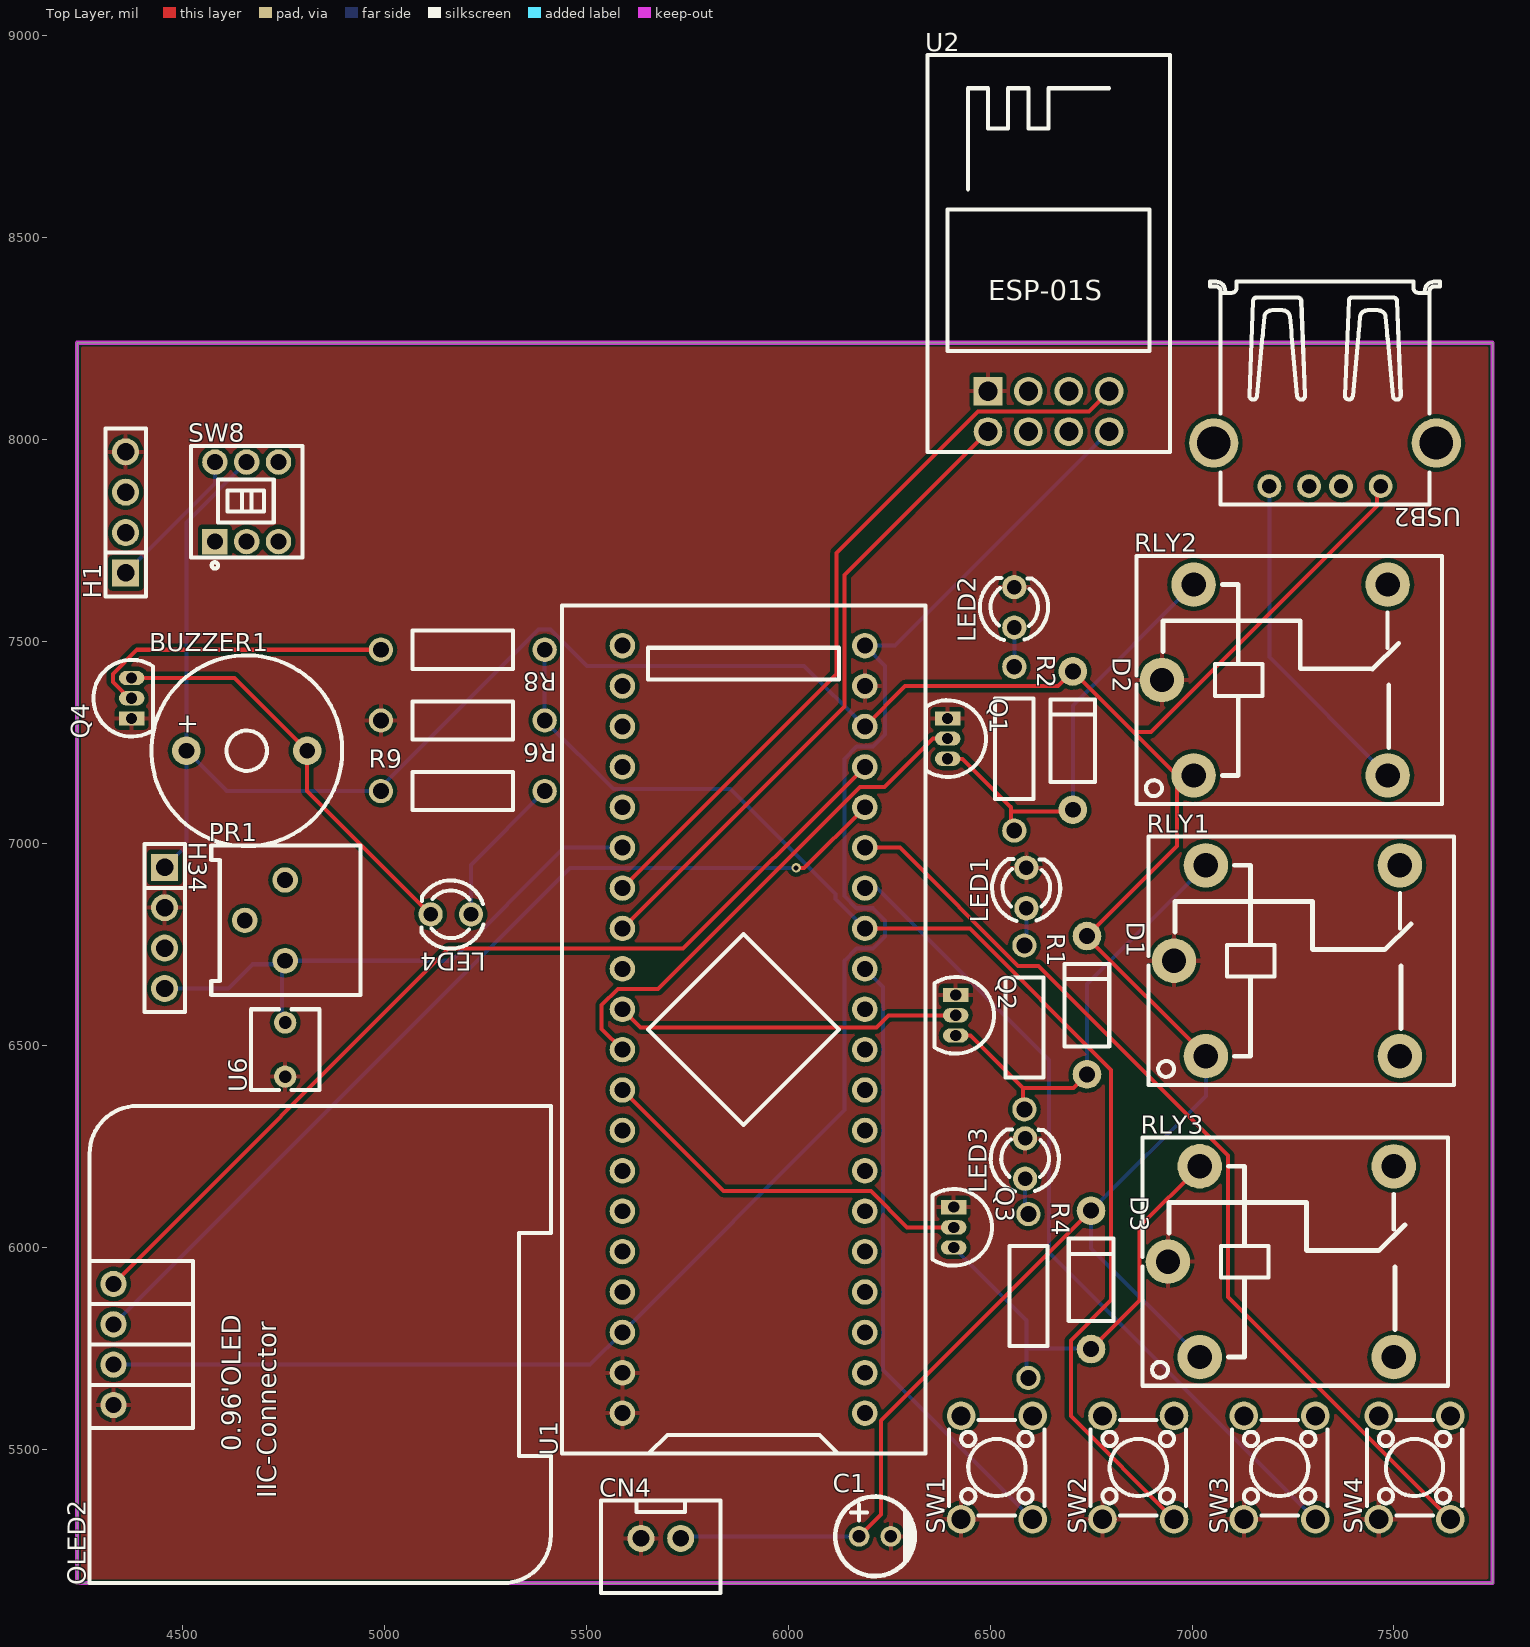
[diagram p0: Top Layer view]
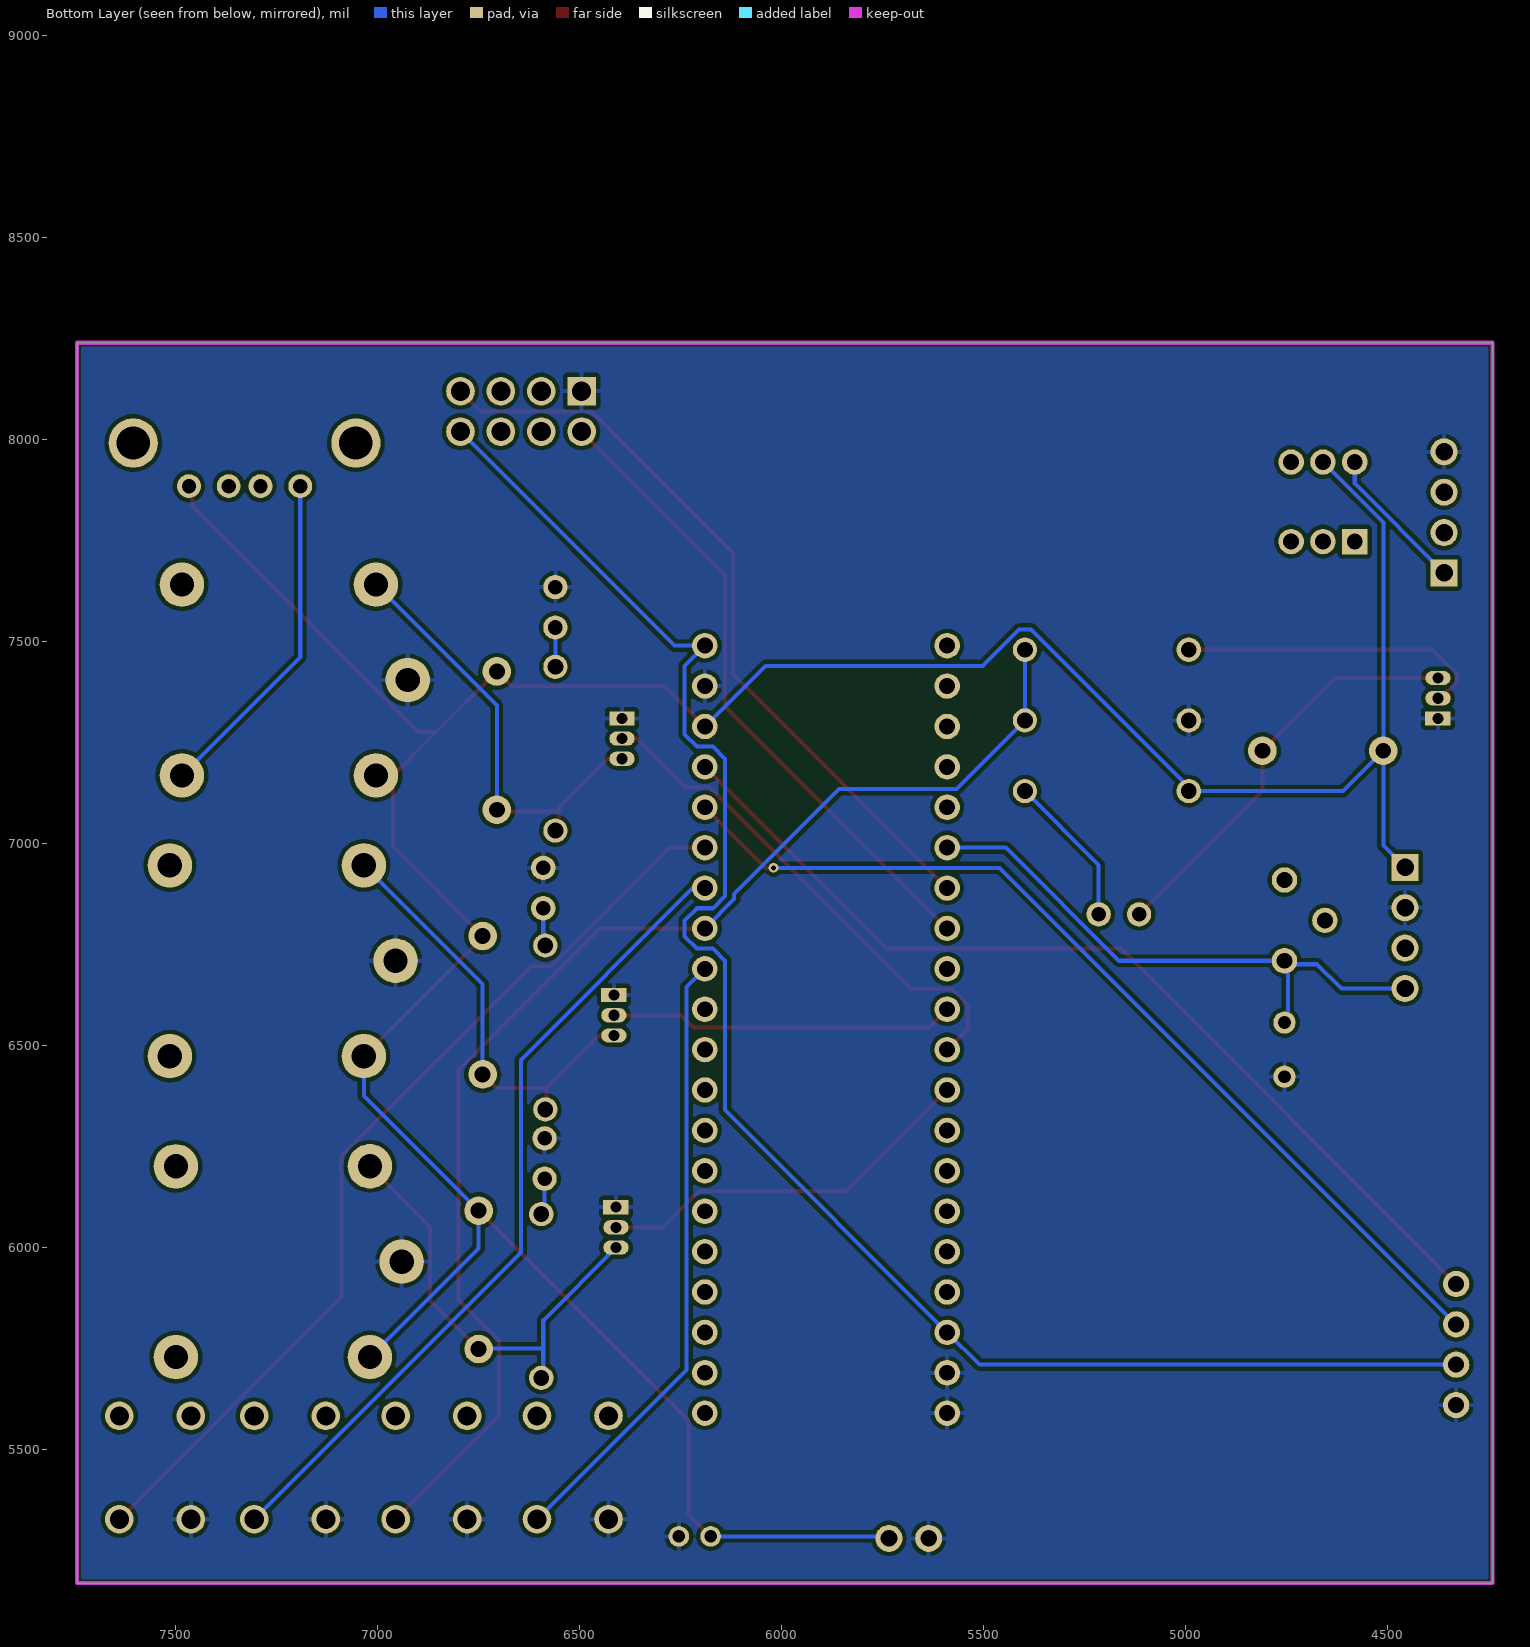
[diagram p1: Bottom Layer view, seen from below]
# Altium PCB MISC51908.pcbdoc
Units mil, origin at the board's own origin, x right, y up, seen from the top; angles counter-clockwise.
Board outline 3503.94 x 3070.87 mil, 2 copper layers (Top Layer, Bottom Layer), stack 62.206 mil thick; 36 components, 50 nets, 152 pads, 1 vias.

## Layer stack, top to bottom
Top Solder Mask Layer: solder mask 0.394, Dk 3.3
Top Layer: signal copper 1.379
Dielectric1: surface 59.449, FR4, Dk 4.5
Bottom Layer: signal copper 1.378
Bottom Solder Mask Layer: solder mask 0.394, Dk 3.3

## Board outline
4240,8240 4240,5169.13 7743.94,5169.13 7743.94,8240

## Design rules (kind name [scope] priority, off if disabled: settings)
BoardOutlineClearance copperThickness2oz_1 [All] p2 off: genericclearance=7.99 ignorepadtopadclearanceinfootprint=FALSE except(0: Arc-SplitContinuation Track-SplitContinuation SMDPad-SplitContinuation THPad-SplitContinuation Via-SplitContinuation Fill-SplitContinuation Region-SplitContinuation Poly-SplitContinuation Text-SplitContinuation Hole-SplitContinuation; 5.98: Arc-CutoutEdge Track-CutoutEdge SMDPad-CutoutEdge THPad-CutoutEdge Via-CutoutEdge Text-CutoutEdge; 6.9: Hole-OutlineEdge Hole-CutoutEdge; 10: Poly-OutlineEdge Poly-CutoutEdge; 11.81: Arc-OutlineEdge Track-OutlineEdge SMDPad-OutlineEdge THPad-OutlineEdge Via-OutlineEdge Fill-OutlineEdge Region-OutlineEdge Text-OutlineEdge Fill-CutoutEdge Region-CutoutEdge)
BoardOutlineClearance Plane_innerPlane_1 [All] p4 off: genericclearance=4.02 ignorepadtopadclearanceinfootprint=FALSE except(0: Arc-SplitContinuation Track-SplitContinuation SMDPad-SplitContinuation THPad-SplitContinuation Via-SplitContinuation Fill-SplitContinuation Region-SplitContinuation Poly-SplitContinuation Text-SplitContinuation Hole-SplitContinuation; 5.98: Arc-CutoutEdge Track-CutoutEdge SMDPad-CutoutEdge THPad-CutoutEdge Via-CutoutEdge Text-CutoutEdge; 6.9: Hole-OutlineEdge Hole-CutoutEdge; 10: Poly-OutlineEdge Poly-CutoutEdge; 11.81: Arc-OutlineEdge Track-OutlineEdge SMDPad-OutlineEdge THPad-OutlineEdge Via-OutlineEdge Fill-OutlineEdge Region-OutlineEdge Text-OutlineEdge Fill-CutoutEdge Region-CutoutEdge)
BoardOutlineClearance Copper_copperRegion_1 [All] p6 off: genericclearance=4.02 ignorepadtopadclearanceinfootprint=FALSE except(0: Arc-SplitContinuation Track-SplitContinuation SMDPad-SplitContinuation THPad-SplitContinuation Via-SplitContinuation Fill-SplitContinuation Region-SplitContinuation Poly-SplitContinuation Text-SplitContinuation Hole-SplitContinuation; 5.98: Arc-CutoutEdge Track-CutoutEdge SMDPad-CutoutEdge THPad-CutoutEdge Via-CutoutEdge Text-CutoutEdge; 6.9: Hole-OutlineEdge Hole-CutoutEdge; 10: Poly-OutlineEdge Poly-CutoutEdge; 11.81: Arc-OutlineEdge Track-OutlineEdge SMDPad-OutlineEdge THPad-OutlineEdge Via-OutlineEdge Fill-OutlineEdge Region-OutlineEdge Text-OutlineEdge Fill-CutoutEdge Region-CutoutEdge)
BoardOutlineClearance Copper_copperRegion_copperThickness1oz_1 [All] p8 off: genericclearance=4.02 ignorepadtopadclearanceinfootprint=FALSE except(0: Arc-SplitContinuation Track-SplitContinuation SMDPad-SplitContinuation THPad-SplitContinuation Via-SplitContinuation Fill-SplitContinuation Region-SplitContinuation Poly-SplitContinuation Text-SplitContinuation Hole-SplitContinuation; 5.98: Arc-CutoutEdge Track-CutoutEdge SMDPad-CutoutEdge THPad-CutoutEdge Via-CutoutEdge Text-CutoutEdge; 6.9: Hole-OutlineEdge Hole-CutoutEdge; 10: Poly-OutlineEdge Poly-CutoutEdge; 11.81: Arc-OutlineEdge Track-OutlineEdge SMDPad-OutlineEdge THPad-OutlineEdge Via-OutlineEdge Fill-OutlineEdge Region-OutlineEdge Text-OutlineEdge Fill-CutoutEdge Region-CutoutEdge)
BoardOutlineClearance Copper_copperRegion_Copper_copperRegion_1 [All] p10 off: genericclearance=4.02 ignorepadtopadclearanceinfootprint=FALSE except(0: Arc-SplitContinuation Track-SplitContinuation SMDPad-SplitContinuation THPad-SplitContinuation Via-SplitContinuation Fill-SplitContinuation Region-SplitContinuation Poly-SplitContinuation Text-SplitContinuation Hole-SplitContinuation; 5.98: Arc-CutoutEdge Track-CutoutEdge SMDPad-CutoutEdge THPad-CutoutEdge Via-CutoutEdge Text-CutoutEdge; 6.9: Hole-OutlineEdge Hole-CutoutEdge; 10: Poly-OutlineEdge Poly-CutoutEdge; 11.81: Arc-OutlineEdge Track-OutlineEdge SMDPad-OutlineEdge THPad-OutlineEdge Via-OutlineEdge Fill-OutlineEdge Region-OutlineEdge Text-OutlineEdge Fill-CutoutEdge Region-CutoutEdge)
BoardOutlineClearance copperThickness1oz_1 [All] p12: genericclearance=4.02 ignorepadtopadclearanceinfootprint=FALSE except(0: Arc-SplitContinuation Track-SplitContinuation SMDPad-SplitContinuation THPad-SplitContinuation Via-SplitContinuation Fill-SplitContinuation Region-SplitContinuation Poly-SplitContinuation Text-SplitContinuation Hole-SplitContinuation; 5.98: Arc-CutoutEdge Track-CutoutEdge SMDPad-CutoutEdge THPad-CutoutEdge Via-CutoutEdge Text-CutoutEdge; 6.9: Hole-OutlineEdge Hole-CutoutEdge; 10: Poly-OutlineEdge Poly-CutoutEdge; 11.81: Arc-OutlineEdge Track-OutlineEdge SMDPad-OutlineEdge THPad-OutlineEdge Via-OutlineEdge Fill-OutlineEdge Region-OutlineEdge Text-OutlineEdge Fill-CutoutEdge Region-CutoutEdge)
Clearance copperThickness2oz [All] p1 off: gap=7.99 ignorepadtopadclearanceinfootprint=FALSE except(5.98: SMDPad-Track SMDPad-SMDPad THPad-Track SMDPad-THPad THPad-THPad Track-Via SMDPad-Via THPad-Via Via-Via Fill-SMDPad Region-SMDPad Fill-THPad Region-THPad Fill-Via Region-Via Fill-Fill Fill-Region Region-Region Arc-Track Arc-SMDPad Arc-THPad Arc-Via Fill-Arc Region-Arc Arc-Arc Text-Track SMDPad-Text Text-THPad Text-Via Fill-Text Region-Text Arc-Text Text-Text; 6.9: Hole-Track Hole-SMDPad Hole-THPad Hole-Via Fill-Hole Region-Hole Hole-Arc Hole-Text; 10: Poly-Track Poly-SMDPad Poly-THPad Poly-Via Poly-Fill Poly-Region Poly-Poly Poly-Arc Poly-Text Poly-Hole; 11.81: Fill-Track Region-Track)
Clearance Plane_innerPlane [All] p3 off: gap=4.02 ignorepadtopadclearanceinfootprint=FALSE except(5.98: SMDPad-Track SMDPad-SMDPad THPad-Track SMDPad-THPad THPad-THPad Track-Via SMDPad-Via THPad-Via Via-Via Fill-SMDPad Region-SMDPad Fill-THPad Region-THPad Fill-Via Region-Via Fill-Fill Fill-Region Region-Region Arc-Track Arc-SMDPad Arc-THPad Arc-Via Fill-Arc Region-Arc Arc-Arc Text-Track SMDPad-Text Text-THPad Text-Via Fill-Text Region-Text Arc-Text Text-Text; 6.9: Hole-Track Hole-SMDPad Hole-THPad Hole-Via Fill-Hole Region-Hole Hole-Arc Hole-Text; 10: Poly-Track Poly-SMDPad Poly-THPad Poly-Via Poly-Fill Poly-Region Poly-Poly Poly-Arc Poly-Text Poly-Hole; 11.81: Fill-Track Region-Track)
Clearance Copper_copperRegion [All] p5 off: gap=4.02 ignorepadtopadclearanceinfootprint=FALSE except(5.98: SMDPad-Track SMDPad-SMDPad THPad-Track SMDPad-THPad THPad-THPad Track-Via SMDPad-Via THPad-Via Via-Via Fill-SMDPad Region-SMDPad Fill-THPad Region-THPad Fill-Via Region-Via Fill-Fill Fill-Region Region-Region Arc-Track Arc-SMDPad Arc-THPad Arc-Via Fill-Arc Region-Arc Arc-Arc Text-Track SMDPad-Text Text-THPad Text-Via Fill-Text Region-Text Arc-Text Text-Text; 6.9: Hole-Track Hole-SMDPad Hole-THPad Hole-Via Fill-Hole Region-Hole Hole-Arc Hole-Text; 10: Poly-Track Poly-SMDPad Poly-THPad Poly-Via Poly-Fill Poly-Region Poly-Poly Poly-Arc Poly-Text Poly-Hole; 11.81: Fill-Track Region-Track)
Clearance Copper_copperRegion_copperThickness1oz [All] p7 off: gap=4.02 ignorepadtopadclearanceinfootprint=FALSE except(5.98: SMDPad-Track SMDPad-SMDPad THPad-Track SMDPad-THPad THPad-THPad Track-Via SMDPad-Via THPad-Via Via-Via Fill-SMDPad Region-SMDPad Fill-THPad Region-THPad Fill-Via Region-Via Fill-Fill Fill-Region Region-Region Arc-Track Arc-SMDPad Arc-THPad Arc-Via Fill-Arc Region-Arc Arc-Arc Text-Track SMDPad-Text Text-THPad Text-Via Fill-Text Region-Text Arc-Text Text-Text; 6.9: Hole-Track Hole-SMDPad Hole-THPad Hole-Via Fill-Hole Region-Hole Hole-Arc Hole-Text; 10: Poly-Track Poly-SMDPad Poly-THPad Poly-Via Poly-Fill Poly-Region Poly-Poly Poly-Arc Poly-Text Poly-Hole; 11.81: Fill-Track Region-Track)
Clearance Copper_copperRegion_Copper_copperRegion [All] p9 off: gap=4.02 ignorepadtopadclearanceinfootprint=FALSE except(5.98: SMDPad-Track SMDPad-SMDPad THPad-Track SMDPad-THPad THPad-THPad Track-Via SMDPad-Via THPad-Via Via-Via Fill-SMDPad Region-SMDPad Fill-THPad Region-THPad Fill-Via Region-Via Fill-Fill Fill-Region Region-Region Arc-Track Arc-SMDPad Arc-THPad Arc-Via Fill-Arc Region-Arc Arc-Arc Text-Track SMDPad-Text Text-THPad Text-Via Fill-Text Region-Text Arc-Text Text-Text; 6.9: Hole-Track Hole-SMDPad Hole-THPad Hole-Via Fill-Hole Region-Hole Hole-Arc Hole-Text; 10: Poly-Track Poly-SMDPad Poly-THPad Poly-Via Poly-Fill Poly-Region Poly-Poly Poly-Arc Poly-Text Poly-Hole; 11.81: Fill-Track Region-Track)
Clearance copperThickness1oz [All] p11: gap=4.02 ignorepadtopadclearanceinfootprint=FALSE except(5.98: SMDPad-Track SMDPad-SMDPad THPad-Track SMDPad-THPad THPad-THPad Track-Via SMDPad-Via THPad-Via Via-Via Fill-SMDPad Region-SMDPad Fill-THPad Region-THPad Fill-Via Region-Via Fill-Fill Fill-Region Region-Region Arc-Track Arc-SMDPad Arc-THPad Arc-Via Fill-Arc Region-Arc Arc-Arc Text-Track SMDPad-Text Text-THPad Text-Via Fill-Text Region-Text Arc-Text Text-Text; 6.9: Hole-Track Hole-SMDPad Hole-THPad Hole-Via Fill-Hole Region-Hole Hole-Arc Hole-Text; 10: Poly-Track Poly-SMDPad Poly-THPad Poly-Via Poly-Fill Poly-Region Poly-Poly Poly-Arc Poly-Text Poly-Hole; 11.81: Fill-Track Region-Track)
DiffPairsRouting differentialPair [All] p1: maxlimit=6 minlimit=6 mostfreqgap=6 toplayer_minwidth=5 toplayer_prefwidth=10 toplayer_maxwidth=100 toplayer_mingap=6 toplayer_prefgap=6 toplayer_maxgap=6 bottomlayer_minwidth=5 bottomlayer_prefwidth=10 bottomlayer_maxwidth=100 bottomlayer_mingap=6 bottomlayer_prefgap=6 bottomlayer_maxgap=6 maxuncoupledlength=10
HoleToHoleClearance otherClearance [All] p1: gap=11.81 allowstackedmicrovias=TRUE
Length netLength [All] p1: minlimit=0 maxlimit=0
PasteMaskExpansion pasteMaskExpansion [All] p1: expansion=0
PlaneConnect innerPlane [All] p1: planeconnectstyle=Relief reliefexpansion=20 reliefentries=4 reliefconductorwidth=10 reliefairgap=10
PolygonConnect copperRegion_copperThickness1oz [All] p1 off: connectstyle=Relief reliefconductorwidth=10 reliefentries=4 polygonreliefangle="90 Angle" airgapwidth=10 via.connectstyle=Relief via.reliefconductorwidth=10 via.reliefentries=4 via.polygonreliefangle="90 Angle" via.airgapwidth=10
PolygonConnect copperRegion_Copper_copperRegion [All] p2 off: connectstyle=Relief reliefconductorwidth=10 reliefentries=4 polygonreliefangle="90 Angle" airgapwidth=10 via.connectstyle=Relief via.reliefconductorwidth=10 via.reliefentries=4 via.polygonreliefangle="90 Angle" via.airgapwidth=10
PolygonConnect copperRegion [(InNet('GND'))] p3: connectstyle=Relief reliefconductorwidth=10 reliefentries=4 polygonreliefangle="90 Angle" airgapwidth=10 via.connectstyle=Relief via.reliefconductorwidth=10 via.reliefentries=4 via.polygonreliefangle="90 Angle" via.airgapwidth=10
RoutingVias viaSize [All] p1: holewidth=12.01 width=24.02 viastyle="Through Hole" minholewidth=11.81 minwidth=19.68 maxholewidth=248.03 maxwidth=393.7
SolderMaskExpansion solderMaskExpansion [IsVia] p1: expansion=-1000 istentingtop=TRUE
SolderMaskExpansion solderMaskExpansion [All] p2: expansion=2 istentingtop=FALSE
Width copperThickness2oz_2 [All] p1 off: maxlimit=100 minlimit=8 preferedwidth=10
Width copperThickness1oz_2 [All] p2: maxlimit=100 minlimit=5 preferedwidth=10

## Components (designator, comment, footprint, x,y, rotation, side; value= is the part's Value field where it differs from the comment)
BUZZER1 "2.3kHz" BUZ-TH_BD12.0-P7.60-D0.6-FD 4660,7230 r0 top
C1 "10uF" CAP-TH_BD5.0-P2.00-D0.8-FD-10UF50VC110GL 6215,5285 r0 top
CN4 "XH2.54*2P_Through-hole" CONN-TH_2P-P2.50-XH2.54-2P 5685,5280 r0 top
D1 "" DO_1N4007 6740,6600 r270 top
D2 "" DO_1N4007 6705,7255 r270 top
D3 "" DO_1N4007 6750,5920 r270 top
H1 "" HDR-TH_4P-P2.54-V-F 4360,7820 r90 top
H34 "" HDR-TH_4P-P2.54-V-F 4456.62,6791.33 r270 top
LED1 "" LED_TH-3mm 6590,6890 r90 top
LED2 "" LED_TH-3mm 6560,7585 r90 top
LED3 "" LED_TH-3mm 6586.72,6220.4 r90 top
LED4 "" LED_TH-3mm 5165,6825 r180 top
OLED2 "" 0.96OLED_4P 4330,5760 r90 top
PR1 "10K" R_3386P 4755,6810 r0 top
Q1 "" S8050_TO_92 6395,7260 r270 top
Q2 "" S8050_TO_92 6415,6575 r270 top
Q3 "" S8050_TO_92 6410,6050 r270 top
Q4 "" S8050_TO_92 4375,7360 r90 top
R1 "1kΩ" Res_1/4W 6585,6545 r270 top
R2 "1kΩ" Res_1/4W 6560,7235 r270 top
R4 "1kΩ" Res_1/4W 6595,5880 r270 top
R6 "1kΩ" Res_1/4W 5194.77,7305 r180 top
R8 "1kΩ" Res_1/4W 5194.77,7480 r180 top
R9 "120" Res_1/4W 5194.77,7130 r0 top
RLY1 "SRD-05VDC-SL-C" RELAY-TH_SRD-XXVDC-XL-C 7235,6710 r0 top
RLY2 "SRD-05VDC-SL-C" RELAY-TH_SRD-XXVDC-XL-C 7205,7405 r0 top
RLY3 "SRD-05VDC-SL-C" RELAY-TH_SRD-XXVDC-XL-C 7220,5965 r0 top
SW1 "" SW-TH_4P-L6.0-W6.0-P4.50-LS6.5 6516.93,5455.3 r90 top
SW2 "" SW-TH_4P-L6.0-W6.0-P4.50-LS6.5 6866.93,5455.3 r90 top
SW3 "" SW-TH_4P-L6.0-W6.0-P4.50-LS6.5 7216.93,5455.3 r90 top
SW4 "" SW-TH_4P-L6.0-W6.0-P4.50-LS6.5 7550.95,5455.3 r90 top
SW8 "TK-6700-1" SW-TH_TK-6700-1 4659.76,7846.23 r0 top
U1 "STM32F103C8T6-Card" CONN-TH_L53.3-W22.9_STM32F103C8T6-CARD 5890,6540 r90 top
U2 "ESP-01S" WIFIM-TH_ESP-01S 6645,8070 r0 top
U6 "光敏电阻-5MM" RES-TH_L4.9-W4.3-P3.4 4755,6490 r90 top
USB2 "" "USB_ Type-A" 7330,8100 r180 top

## Footprints (in the part's own frame and the unit in brackets; to place one, negate y for a bottom-side part, rotate by r counter-clockwise, add the part's x,y. Pads: shape width x height; smd on the part's side, far side on the other; paste and mask are expansions set on the pad)
0.96OLED_4P [mm]
  round 1.65 hole 1 copper offset 0,0: 1(-3.81,-0.001) 2(-1.27,0.002) 3(1.27,0.002) 4(3.81,0.002)
  silkscreen extent -15,-27.5 15,1.5
BUZ-TH_BD12.0-P7.60-D0.6-FD [mm]
  round 1.8 hole 1: 1(-3.8,0) 2(3.8,0)
  silkscreen extent -6,-6 6,6
CAP-TH_BD5.0-P2.00-D0.8-FD-10UF50VC110GL [mm]
  round 1.3 hole 0.8: 1(-1,0) 2(1,0)
  silkscreen extent -2.5,-2.5 2.5,2.5
CONN-TH_2P-P2.50-XH2.54-2P [mm]
  round 1.7 hole 1.05 paste+0 mask+0.05: 1(1.25,0) 2(-1.25,0)
  silkscreen extent -3.75,-3.42 3.75,2.37
CONN-TH_L53.3-W22.9_STM32F103C8T6-CARD [mm]
  round 1.6 hole 1: 1(-24.13,-7.62) 2(-21.59,-7.62) 3(-19.05,-7.62) 4(-16.51,-7.62) 5(-13.97,-7.62) 6(-11.43,-7.62) 7(-8.89,-7.62) 8(-6.35,-7.62) 9(-3.81,-7.62) 10(-1.27,-7.62) 11(1.27,-7.62) 12(3.81,-7.62) 13(6.35,-7.62) 14(8.89,-7.62) 15(11.43,-7.62) 16(13.97,-7.62) 17(16.51,-7.62) 18(19.05,-7.62) 19(21.59,-7.62) 20(24.13,-7.62) 21(24.13,7.62) 22(21.59,7.62) 23(19.05,7.62) 24(16.51,7.62) 25(13.97,7.62) 26(11.43,7.62) 27(8.89,7.62) 28(6.35,7.62) 29(3.81,7.62) 30(1.27,7.62) 31(-1.27,7.62) 32(-3.81,7.62) 33(-6.35,7.62) 34(-8.89,7.62) 35(-11.43,7.62) 36(-13.97,7.62) 37(-16.51,7.62) 38(-19.05,7.62) 39(-21.59,7.62) 40(-24.13,7.62)
  silkscreen extent -26.67,-11.43 26.67,11.43
DO_1N4007 [mm]
  round 1.8 hole 1 paste+0 mask+0.051: 1(-4.35,0) 2(4.35,0)
  silkscreen extent -2.6,-1.4 2.6,1.4
HDR-TH_4P-P2.54-V-F [mm]
  rect 1.7x1.7 hole 1.1: 1(-3.81,0)
  round 1.7 hole 1.1: 2(-1.27,0) 3(1.27,0) 4(3.81,0)
  silkscreen extent -5.29,-1.27 5.29,1.27
LED_TH-3mm [mil]
  round 60 hole 36 paste+0 mask+2: 1(-50,0) 2(50,0)
  silkscreen extent -81,-84 72,85
R_3386P [mil]
  round 63 hole 39.4 paste+0 mask+2: 1(0,-100) 2(-100,0) 3(0,100)
  silkscreen extent -183,-185 187,185
RELAY-TH_SRD-XXVDC-XL-C [mil]
  round 110 hole 60: 1(-200.79,-236.22) 2(279.52,-236.2) 3(279.53,236.2) 4(-200.79,236.22) 5(-279.53,0)
  silkscreen extent -342,-307 413,307
RES-TH_L4.9-W4.3-P3.4 [mm]
  round 1.4 hole 0.8 paste+0 mask+0.05: 1(-1.7,0) 2(1.7,0)
  silkscreen extent -2.54,-2.16 2.54,2.16
Res_1/4W [mil]
  round 60 hole 39.37 paste+0 mask+2: 1(-202.76,0) 2(202.76,0)
  silkscreen extent -124,-47 124,47
S8050_TO_92 [mil]
  rect 35.4x63 hole 27.6 paste+0 mask+2: 1(-50,0)
  oval 35.4x63 hole 27.6 paste+0 mask+2: 2(0,0) 3(50,0)
  silkscreen extent -95,-53 95,95
SW-TH_4P-L6.0-W6.0-P4.50-LS6.5 [mm]
  round 1.8 hole 1.2: 1(-3.25,2.25) 2(3.25,2.25) 3(-3.25,-2.25) 4(3.25,-2.25)
  silkscreen extent -3,-3 3,3
SW-TH_TK-6700-1 [mm]
  rect 1.6x1.6 hole 1 paste+0 mask+0.051: 1(-2,-2.5)
  round 1.6 hole 1 paste+0 mask+0.051: 2(0,-2.5) 3(2,-2.5)
  round 1.6 hole 1 copper offset 0,0 paste+0 mask+0.051: 4(-2,2.5) 5(0,2.5) 6(2,2.5)
  silkscreen extent -3.5,-4.2 3.5,3.5
"USB_ Type-A" [mm]
  round 1.5 hole 0.9 copper offset 0,0 paste+0 mask+0.051: 1(-3.484,5.461) 4(3.516,5.461)
  round 1.5 hole 0.9 paste+0 mask+0.051: 2(-0.984,5.461) 3(1.016,5.461)
  round 3.1 hole 2.1 paste+0 mask+0.051: SH1(7.016,2.751) SH2(-6.984,2.751)
  silkscreen extent -7.2,-7.4 7.24,6.6
WIFIM-TH_ESP-01S [mm]
  rect 1.8x1.8 hole 1.2: 1(-3.81,1.27)
  round 1.8 hole 1.2: 2(-1.27,1.27) 3(1.27,1.27) 4(3.81,1.27) 5(3.81,-1.27) 6(1.27,-1.27) 7(-1.27,-1.27) 8(-3.81,-1.27)
  silkscreen extent -7.62,-2.54 7.62,22.4

## Via types
v1: diameter 24.02, hole 12, Top Layer to Bottom Layer, 1 vias

## Nets (pads, with @x,y where several pads share a name; then routed paths per layer and width w, separated by ;. In a path a pad name is that pad's centre, name@x,y a point inside that pad or via, vN(x,y) a via of type N, cw(c..) or ccw(c..) an arc to the next point about the centre after c; other vN are vias at no path point)
3V3: PR1.2
$1N17203: LED1.1 R1.1 | length 94.3
  Bottom Layer w10: R1.1 6590,6752.76 LED1.1
$1N17204: D1.2 Q2.3 R1.2 RLY1.4 | length 1086.4
  Top Layer w10: Q2.3 6451.5,6525 6581.5,6395 ; R1.2 6581.5,6345.74 6581.5,6395 ; D1.2 6706.26,6395 6581.5,6395
  Bottom Layer w10: D1.2 6740,6652.01 RLY1.4
$1N17207: D2.2 Q1.3 R2.2 RLY2.4 | length 1103.9
  Top Layer w10: Q1.3 6431.5,7210 6551.5,7090 6551.5,7080 ; R2.2 6551.5,7040.74 6551.5,7080 ; D2.2 6701.26,7080 6551.5,7080
  Bottom Layer w10: D2.2 6705,7342.01 RLY2.4
$1N17208: LED2.1 R2.1 | length 97.2
  Bottom Layer w10: R2.1 LED2.1
$1N17214: RLY2.2 USB2.4 | length 837.5
  Bottom Layer w10: USB2.4 7191.58,7461.75 RLY2.2
$1N17217: D3.2 Q3.3 R4.2 RLY3.4 | length 1123.9
  Top Layer w10: D3.2 6870,5868.74 6870,6052.01 RLY3.4
  Bottom Layer w10: Q3.3 6590,5820 6590,5750 ; R4.2 6590,5682.24 6590,5750 ; D3.2 6748.74,5750 6590,5750
$1N17218: LED3.1 R4.1 | length 91.1
  Bottom Layer w10: LED3.1 6586.72,6091.04 R4.1
$1N17224: RLY3.2
$1N17232: LED4.1 R9.2 | length 380.6
  Bottom Layer w10: LED4.1 5215,6947.47 R9.2
$1N17233: Q4.2 R8.2 | length 771.4
  Top Layer w10: Q4.2 4368.5,7360 4328.5,7400 4328.5,7420 4388.5,7480 R8.2
$1N17237: BUZZER1.2 LED4.2 Q4.3 | length 1040.7
  Top Layer w10: Q4.3 4629.61,7410 BUZZER1.2 4809.61,7130.39 LED4.2
+5V: BUZZER1.1 C1.1 CN4.1 D1.1 D2.1 D3.1 H34.1 R9.1 RLY1.1 RLY2.1 RLY3.1 SW8.5 U1.18 USB2.1 | length 8315.4
  Top Layer w10: C1.1 6230,5339.37 6230,5571.26 D3.1 ; U1.18 6290,7390 6668.74,7390 D2.1 6855,7276.26 ; RLY2.1 RLY2.1@6962.48,7168.78 ; RLY1.1 6740,6767.99 D1.1 6962.48,6993.74 RLY2.1@6962.48,7168.78 ; USB2.1 7458.43,7876.26 7458.43,7836.26 6898.43,7276.26 6855,7276.26 ; 6855,7276.26 RLY2.1@6962.48,7168.78
  Bottom Layer w10: H34.1 4510.39,6995.11 BUZZER1.1 ; SW8.5 4510.39,7795.28 BUZZER1.1 ; CN4.1 5739.22,5285 C1.1 ; U1.18 6040,7440 5502.01,7440 5412.01,7530 5382.01,7530 4992.01,7140 R9.1 4610.39,7130 BUZZER1.1 ; RLY3.1 6750,5997.99 D3.1 7034.21,6375.47 RLY1.1
GND: C1.2 CN4.2 H1.4 H34.2 LED1.2 LED2.2 LED3.2 OLED2.1 Q1.1 Q2.1 Q3.1 Q4.1 R6.2 RLY1.5 RLY2.5 RLY3.5 SW1.1 SW2.1 SW3.1 SW4.1 U1.19 U1.39 U1.40 U2.1 U6.1
NRST: U1.37
PA0: U1.25
PA1: H34.4 PR1.1 U1.26 U6.2 | length 1425.8
  Bottom Layer w10: H34.4 4614.1,6641.33 4674.1,6701.33 PR1.1@4746.62,6701.33 ; U6.2 4746.62,6565.31 PR1.1@4746.62,6701.33 ; U1.26 5445,6990 5165,6710 PR1.1 PR1.1@4746.62,6701.33
PA2: U1.27 U2.4 | length 1890.2
  Top Layer w10: U1.27 6120,7420 6120,7720 6470,8070 6745,8070 U2.4
PA3: U1.28 U2.8 | length 1604.9
  Top Layer w10: U1.28 6140,7340 6140,7665 U2.8
PA4: U1.29
PA5: Q2.2 U1.30 | length 856.1
  Top Layer w10: U1.30 5635.01,6545 6218.5,6545 6248.5,6575 Q2.2
PA6: Q1.2 U1.31 | length 1261.2
  Top Layer w10: U1.31 5538.5,6541.5 5538.5,6600 5578.5,6640 5678.5,6640 6178.5,7140 6238.5,7140 6358.5,7260 Q1.2
PA7: Q3.2 U1.32 | length 960.8
  Top Layer w10: U1.32 5840,6140 6204.76,6140 6294.76,6050 Q3.2
PA8: U1.5
PA9: U1.6
PA10: U1.7
PA11: U1.8
PA12: U1.9
PA15: U1.10
PB0: U1.33
PB1: U1.34
PB3: U1.11
PB4: SW1.3 U1.12 | length 1534.8
  Bottom Layer w10: U1.12 6235.51,6644.5 6235.51,5697.35 SW1.3
PB5: R6.1 R8.1 SW2.3 U1.13 | length 3203
  Top Layer w10: U1.13 6450,6790 6800,6440.01 6800,5870.01 6700,5770.01 6700,5582.86 SW2.3
  Bottom Layer w10: R8.1 R6.1 5567.53,7135 5857.52,7135 6117.52,6875 6117.52,6862.48 U1.13
PB6: SW3.3 U1.14 | length 2042.3
  Bottom Layer w10: U1.14 6220,6890 6645.51,6464.49 6645.51,5987.35 SW3.3
PB7: SW4.3 U1.15 | length 2343.2
  Top Layer w10: U1.15 6276.87,6990 6569.53,6697.35 6619.53,6697.35 7089.53,6227.35 7089.53,5877.35 SW4.3
PB8: OLED2.3 U1.16 | length 2390.2
  Top Layer w10: v1(6019.95,6940) 6039.99,6940 U1.16
  Bottom Layer w10: OLED2.3 5459.95,6940 v1(6019.95,6940)
PB9: OLED2.4 U1.17 | length 2390.2
  Top Layer w10: OLED2.4 5159.95,6740 5739.99,6740 U1.17
PB10: U1.35
PB11: U1.36
PB12: U1.1
PB13: U1.2
PB14: U1.3
PB15: U1.4
PC13: U1.22
PC14: U1.23
PC15: U1.24
VBAT: U1.21
VCC: OLED2.2 U1.20 U1.38 U2.5 | length 4260.8
  Bottom Layer w10: OLED2.2 5510,5710 U1.38 6140,6340 6140,6710 6170,6740 6210,6740 6240,6770 6240,6810 6210,6840 6170,6840 6140,6870 6140,7210 6170,7240 6210,7240 6240,7270 6240,7440 U1.20 6265,7490 U2.5
VUSB: H1.1 SW8.4 | length 366.2
  Bottom Layer w10: H1.1 4581.02,7891.02 SW8.4
pads on no net: H1.2 H1.3 H34.3 PR1.3 RLY1.2 RLY1.3 RLY2.3 RLY3.3 SW1.2 SW1.4 SW2.2 SW2.4 SW3.2 SW3.4 SW4.2 SW4.4 SW8.1 SW8.2 SW8.3 SW8.6 U2.2 U2.3 U2.6 U2.7 USB2.2 USB2.3 USB2.SH1 USB2.SH2

## Polygon pours and split planes (outlines as drawn)
GND on Top Layer (solid, remove dead copper, pour order 0): 3000,10100 3000,3000 8985,3000 8985,10100
GND on Bottom Layer (solid, remove dead copper, pour order 2): 3085,9625 3085,4305 8400,4305 8400,9625

## Keep-outs
Board Outline Layer:
  the board outline again, w10